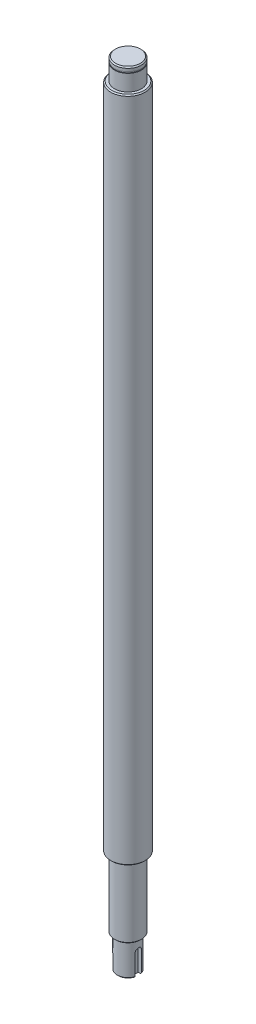
from build123d import *

# Parameters (mm, degrees)
SKETCH_5_W          = 16
SKETCH_5_H          = 619
SKETCH_6_R          = 12.5
EXTRUDE_1_DEPTH     = 65
SKETCH_7_R          = 10
EXTRUDE_2_DEPTH     = 30
EXTRUDE_START       = 20
SKETCH_8_R          = 12.5
EXTRUDE_3_DEPTH     = 20
SKETCH_9_W          = 13.903089526
SKETCH_9_H          = 1.35
CHAMFER_1_SIZE      = 1
CUT_EXTRUDE_1_DEPTH = 3.5


with BuildPart() as part:
    # 草图5 → 旋转2 (revolve)
    with BuildSketch(Plane(origin=(0, 0, 0), x_dir=(-1, 0, 0), z_dir=(0, 0, -1)), mode=Mode.PRIVATE) as revolve_2_sk:
        with Locations((-8, 15)):
            Rectangle(SKETCH_5_W, SKETCH_5_H)
    revolve(revolve_2_sk.sketch.rotate(Axis((0, -294.5, 0), (0, 1, 0)), 270), axis=Axis((0, -294.5, 0), (0, 1, 0)))

    # 草图6 → 凸台-拉伸1 (add)
    with BuildSketch(Plane.XZ.offset(294.5)):
        with Locations(Location((0, 0, 0), (0, 0, 270))):
            Circle(SKETCH_6_R)
    extrude(amount=EXTRUDE_1_DEPTH)

    # 草图7 → 凸台-拉伸2 (add)
    with BuildSketch(Plane.XZ.offset(359.5)):
        with Locations(Location((0, 0, 0), (0, 0, 270))):
            Circle(SKETCH_7_R)
    extrude(amount=EXTRUDE_2_DEPTH)

    # 草图8 → 凸台-拉伸3 (add)
    with BuildSketch(Plane(origin=(0, 324.5, 0), x_dir=(1, 0, 0), z_dir=(0, 1, 0)).offset(EXTRUDE_START)):
        with Locations(Location((0, 0, 0), (0, 0, 90))):
            Circle(SKETCH_8_R)
    extrude(amount=-EXTRUDE_3_DEPTH)

    # 草图9 → 切除-旋转1 (revolve, cut)
    with BuildSketch(Plane(origin=(0, 0, 0), x_dir=(-1, 0, 0), z_dir=(0, 0, -1)), mode=Mode.PRIVATE) as cut_revolve_1_sk:
        with Locations((18.901544763, 340.175)):
            Rectangle(SKETCH_9_W, SKETCH_9_H)
    revolve(cut_revolve_1_sk.sketch.rotate(Axis((0, 0, 0), (0, 1, 0)), 270), axis=Axis((0, 0, 0), (0, 1, 0)), mode=Mode.SUBTRACT)

    # 倒角1
    chamfer_1_edges = [part.edges().sort_by_distance(p)[0] for p in [
        (0, -359.5, 12.5),
        (0, -389.5, 10),
        (0, 344.5, 12.5),
        (0, 324.5, -16),
        (0, -294.5, -16),
    ]]
    chamfer(chamfer_1_edges, length=CHAMFER_1_SIZE)

    # 草图10 → 切除-拉伸1 (cut)
    with BuildSketch(Plane(origin=(10, 0, 0), x_dir=(0, 0, -1), z_dir=(1, 0, 0))):
        with BuildLine():
            Line((3, -369.5), (3, -402.553548126))
            ThreePointArc((3, -402.553548126), (0, -405.553548126), (-3, -402.553548126))
            Line((-3, -402.553548126), (-3, -369.5))
            ThreePointArc((-3, -369.5), (0, -366.5), (3, -369.5))
        make_face()
    extrude(amount=-CUT_EXTRUDE_1_DEPTH, mode=Mode.SUBTRACT)


solid = part.part
